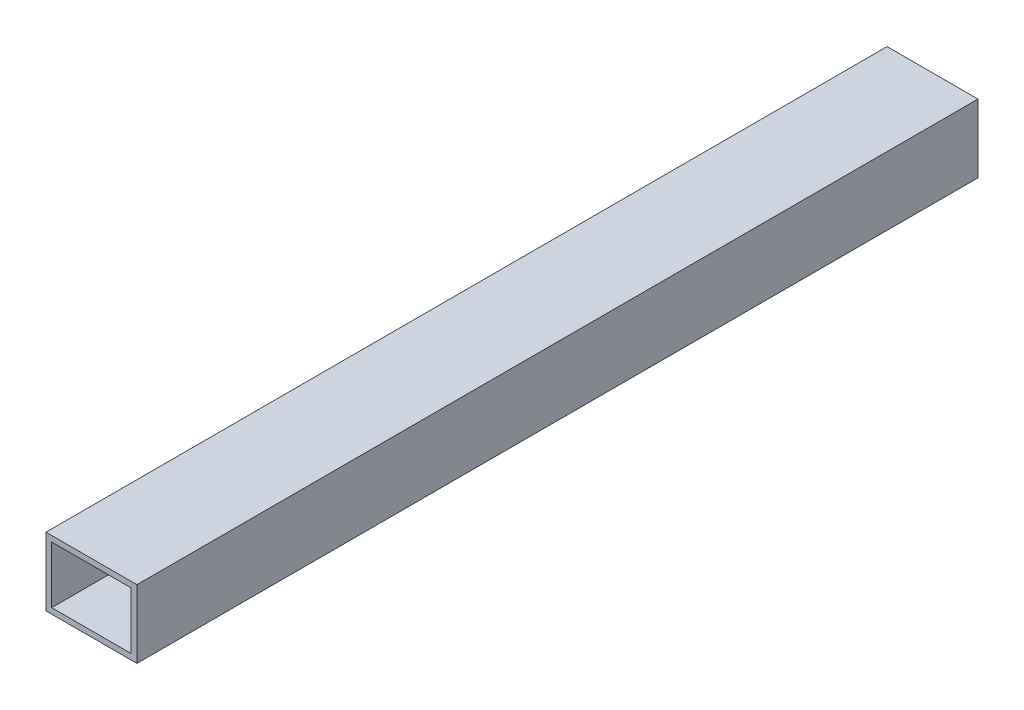
SolidWorks part; units mm, degrees
ref_plane "前视基准面" through (0, 0, 0) normal (0, 0, 1) x (1, 0, 0)
ref_plane "上视基准面" through (0, 0, 0) normal (0, 1, 0) x (1, 0, 0)
ref_plane "右视基准面" through (0, 0, 0) normal (1, 0, 0) x (0, 0, -1)
sketch "草图1" plane through (0, 0, 0) normal (0, 0, 1) x (1, 0, 0)
  line L0 (0, 0) -> (80, 0)
  line L1 (80, 0) -> (80, -60)
  line L2 (80, -60) -> (0, -60)
  line L3 (0, -60) -> (0, 0)
  line L4 (3, -3) -> (77, -3)
  line L5 (77, -3) -> (77, -57)
  line L6 (77, -57) -> (3, -57)
  line L7 (3, -57) -> (3, -3)
  dimension "D1" = 3
extrude "凸台-拉伸1" add sketch "草图1" along normal blind 740
sketch "草图2" plane through (0, 0, 0) normal (0, 1, 0) x (1, 0, 0)
  line L0 (0, -370) -> (80, -370)
  line L1 (0, -740) -> (0, 0) construction
  line L2 (80, -740) -> (80, 0) construction
sketch "草图3" plane through (0, 0, 740) normal (0, 0, 1) x (1, 0, 0)
  line L8 (0, 0) -> (0, -60)
  line L9 (0, -60) -> (80, -60)
  line L10 (80, -60) -> (80, 0)
  line L11 (80, 0) -> (0, 0)
  line L12 (0, 0) -> (0, -60)
  line L13 (0, -60) -> (80, -60)
  line L14 (80, -60) -> (80, 0)
  line L15 (80, 0) -> (0, 0)
  dimension "D1" = 0
extrude "切除-拉伸1" cut sketch "草图3" against normal blind 25
sketch "草图4" plane through (0, 0, 0) normal (0, 0, -1) x (-1, 0, 0)
  line L8 (0, -60) -> (0, 0)
  line L9 (0, 0) -> (-80, 0)
  line L10 (-80, 0) -> (-80, -60)
  line L11 (-80, -60) -> (0, -60)
  line L12 (0, -60) -> (0, 0)
  line L13 (0, 0) -> (-80, 0)
  line L14 (-80, 0) -> (-80, -60)
  line L15 (-80, -60) -> (0, -60)
  dimension "D1" = 0
extrude "切除-拉伸2" cut sketch "草图4" against normal blind 25
sketch "草图5" plane through (0, 0, 715) normal (0, 0, 1) x (1, 0, 0)
  line L4 (3, -3) -> (3, -57)
  line L5 (3, -57) -> (77, -57)
  line L6 (77, -57) -> (77, -3)
  line L7 (77, -3) -> (3, -3)
  line L8 (80, 0) -> (0, 0)
  line L9 (0, 0) -> (0, -60)
  line L10 (0, -60) -> (80, -60)
  line L11 (80, -60) -> (80, 0)
  line L12 (80, 0) -> (0, 0)
  line L13 (0, 0) -> (0, -60)
  line L14 (0, -60) -> (80, -60)
  line L15 (80, -60) -> (80, 0)
  dimension "D1" = 0
extrude "凸台-拉伸2" add sketch "草图5" along normal blind 25
sketch "草图6" plane through (0, 0, 25) normal (0, 0, -1) x (-1, 0, 0)
  line L8 (-77, -3) -> (-77, -57)
  line L9 (-77, -57) -> (-3, -57)
  line L10 (-3, -57) -> (-3, -3)
  line L11 (-3, -3) -> (-77, -3)
  line L12 (-80, -60) -> (0, -60)
  line L13 (0, -60) -> (0, 0)
  line L14 (0, 0) -> (-80, 0)
  line L15 (-80, 0) -> (-80, -60)
  line L16 (-80, -60) -> (0, -60)
  line L17 (0, -60) -> (0, 0)
  line L18 (0, 0) -> (-80, 0)
  line L19 (-80, 0) -> (-80, -60)
  dimension "D1" = 0
extrude "凸台-拉伸3" add sketch "草图6" along normal blind 25
sketch "草图7" plane through (80, 0, 0) normal (1, 0, 0) x (0, 0, -1)
  line L0 (-740, -60) -> (-740, -55)
  line L1 (-740, -60) -> (-740, 0) construction
  line L2 (-740, -55) -> (-695, -55)
  line L3 (-695, -55) -> (-695, -60)
  line L4 (-740, -60) -> (0, -60) construction
  line L5 (-695, -60) -> (-740, -60)
  line L6 (0, -60) -> (0, -55)
  line L7 (0, 0) -> (0, -60) construction
  line L8 (0, -55) -> (-45, -55)
  line L9 (-45, -55) -> (-45, -60)
  line L10 (-45, -60) -> (0, -60)
extrude "切除-拉伸3" cut sketch "草图7" against normal blind 80
sketch "草图8" plane through (0, 0, 45) normal (0, 0, -1) x (-1, 0, 0)
  line L16 (-3, -55) -> (-3, -57)
  line L17 (-3, -57) -> (-77, -57)
  line L18 (-77, -57) -> (-77, -55)
  line L19 (-77, -55) -> (-80, -55)
  line L20 (-80, -55) -> (-80, -60)
  line L21 (-80, -60) -> (0, -60)
  line L22 (0, -60) -> (0, -55)
  line L23 (0, -55) -> (-3, -55)
  line L24 (-3, -55) -> (-3, -57)
  line L25 (-3, -57) -> (-77, -57)
  line L26 (-77, -57) -> (-77, -55)
  line L27 (-77, -55) -> (-80, -55)
  line L28 (-80, -55) -> (-80, -60)
  line L29 (-80, -60) -> (0, -60)
  line L30 (0, -60) -> (0, -55)
  line L31 (0, -55) -> (-3, -55)
  dimension "D1" = 0
extrude "凸台-拉伸4" add sketch "草图8" along normal blind 45
sketch "草图9" plane through (0, 0, 695) normal (0, 0, 1) x (1, 0, 0)
  line L16 (3, -57) -> (3, -55)
  line L17 (3, -55) -> (0, -55)
  line L18 (0, -55) -> (0, -60)
  line L19 (0, -60) -> (80, -60)
  line L20 (80, -60) -> (80, -55)
  line L21 (80, -55) -> (77, -55)
  line L22 (77, -55) -> (77, -57)
  line L23 (77, -57) -> (3, -57)
  line L24 (3, -57) -> (3, -55)
  line L25 (3, -55) -> (0, -55)
  line L26 (0, -55) -> (0, -60)
  line L27 (0, -60) -> (80, -60)
  line L28 (80, -60) -> (80, -55)
  line L29 (80, -55) -> (77, -55)
  line L30 (77, -55) -> (77, -57)
  line L31 (77, -57) -> (3, -57)
  dimension "D1" = 0
extrude "凸台-拉伸5" add sketch "草图9" along normal blind 45
sketch "草图10" plane through (0, 0, 0) normal (0, 0, -1) x (-1, 0, 0)
  line L2 (-3, -3) -> (-77, -3)
  line L3 (-3, -3) -> (-77, -3)
  line L5 (-77, -3) -> (-77, -57)
  line L6 (-77, -3) -> (-77, -57)
  line L8 (-3, -57) -> (-3, -3)
  line L9 (-3, -57) -> (-3, -3)
  line L10 (-5, -55) -> (-5, -5)
  line L11 (-3, -57) -> (-77, -57)
  line L12 (-3, -57) -> (-77, -57)
  line L13 (-5, -5) -> (-75, -5)
  line L14 (-75, -5) -> (-75, -55)
  line L15 (-5, -55) -> (-75, -55)
  dimension "D1" = 0
  dimension "D2" = 0
  dimension "D3" = 0
  dimension "D4" = 0
  dimension "D5" = 2
extrude "凸台-拉伸6" add sketch "草图10" against normal blind 740
